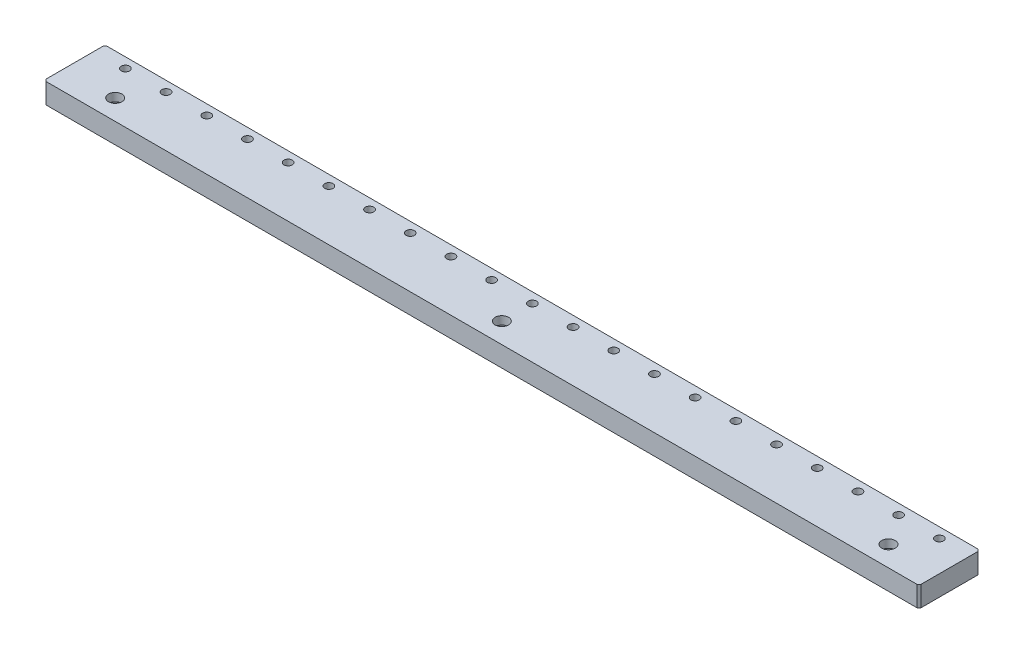
SolidWorks part; units mm, degrees
material "A6061"
ref_plane "前基準面" through (0, 0, 0) normal (0, 0, 1) x (1, 0, 0)
ref_plane "上基準面" through (0, 0, 0) normal (0, 1, 0) x (1, 0, 0)
ref_plane "右基準面" through (0, 0, 0) normal (1, 0, 0) x (0, 0, -1)
sketch "草图1" plane through (0, 0, 0) normal (0, 1, 0) x (1, 0, 0)
  line L1 (-215, -15) -> (215, -15)
  line L2 (-215, -15) -> (-215, 15)
  line L3 (-215, 15) -> (215, 15)
  line L4 (215, -15) -> (215, 15)
  line L5 (-215, -15) -> (215, 15) construction
  line L6 (-215, 15) -> (215, -15) construction
  point P0 (0, 0)
  dimension "D1" = 430
  dimension "D2" = 30
extrude "凸台-拉伸1" add sketch "草图1" along normal mid plane 10
chamfer "倒角1" distance 1 angle 45 4 edges at (-215, 0, 15) (-215, 0, -15) (215, 0, -15) (215, 0, 15)
hole_wizard "打孔尺寸(%根据)内六角圆柱头螺钉的类型1" positions "草图2" profile "草图3" counterbore size "M6" standard "GB" end condition through all
sketch "草图2" plane through (0, -5, 0) normal (0, -1, 0) x (-1, 0, 0)
  line L1 (214, -15) -> (-214, -15) construction
  point P0 (-190, -5)
  point P5 (0, -5)
  point P6 (190, -5)
  dimension "D2" = 190
  dimension "D3" = 10
  dimension "D1" = 3
sketch "草图3" plane through (190, -5, 5) normal (1, 0, 0) x (0, 0, -1)
  line L0 (0, 0) -> (0, 10)
  line L1 (0, 10) -> (3.3, 10)
  line L3 (3.3, 10) -> (3.3, 6)
  line L4 (3.3, 6) -> (5.5, 6)
  line L5 (5.5, 6) -> (5.5, 0)
  line L7 (5.5, 0) -> (0, 0)
  line L11 (0, -6.35) -> (0, 107.95) construction
  dimension "通孔孔直径" = 6.6
  dimension "通孔孔深度" = 10
  dimension "柱形沉头孔直径" = 11
  dimension "柱形沉头孔深度" = 6
hole_wizard "Ø4.1 (4.1) 直径孔1" positions "草图4" profile "草图5" hole size "Ø4.1" standard "GB"
sketch "草图4" plane through (0, -5, -18.75) normal (0, 1, 0) x (-1, 0, 0)
  line L0 (214, 33.75) -> (-214, 33.75) construction
  line L1 (0, 33.75) -> (0, -31.8683) construction
  point P0 (-200, 8.75)
  point P5 (-180, 8.75)
  point P6 (-160, 8.75)
  point P7 (-140, 8.75)
  point P8 (-120, 8.75)
  point P9 (-100, 8.75)
  point P10 (-80, 8.75)
  point P11 (-60, 8.75)
  point P12 (-40, 8.75)
  point P13 (-20, 8.75)
  point P14 (0, 8.75)
  point P15 (20, 8.75)
  point P16 (40, 8.75)
  point P17 (60, 8.75)
  point P18 (80, 8.75)
  point P19 (100, 8.75)
  point P20 (120, 8.75)
  point P21 (140, 8.75)
  point P22 (160, 8.75)
  point P23 (180, 8.75)
  point P40 (200, 8.75)
  dimension "D2" = 20
  dimension "D3" = 25
  dimension "D1" = 21
sketch "草图5" plane through (200, -5, -10) normal (1, 0, 0) x (0, 0, -1)
  line L0 (0, 0) -> (0, 11.2318)
  line L1 (0, 11.2318) -> (2.05, 10)
  line L2 (2.05, 10) -> (2.05, 0)
  line L5 (2.05, 0) -> (0, 0)
  line L10 (0, 11.2318) -> (-2.05, 10) construction
  line L11 (0, -6.35) -> (0, 107.95) construction
  dimension "孔直径" = 4.1
  dimension "孔深度" = 10
  dimension "导头角度" = 118
